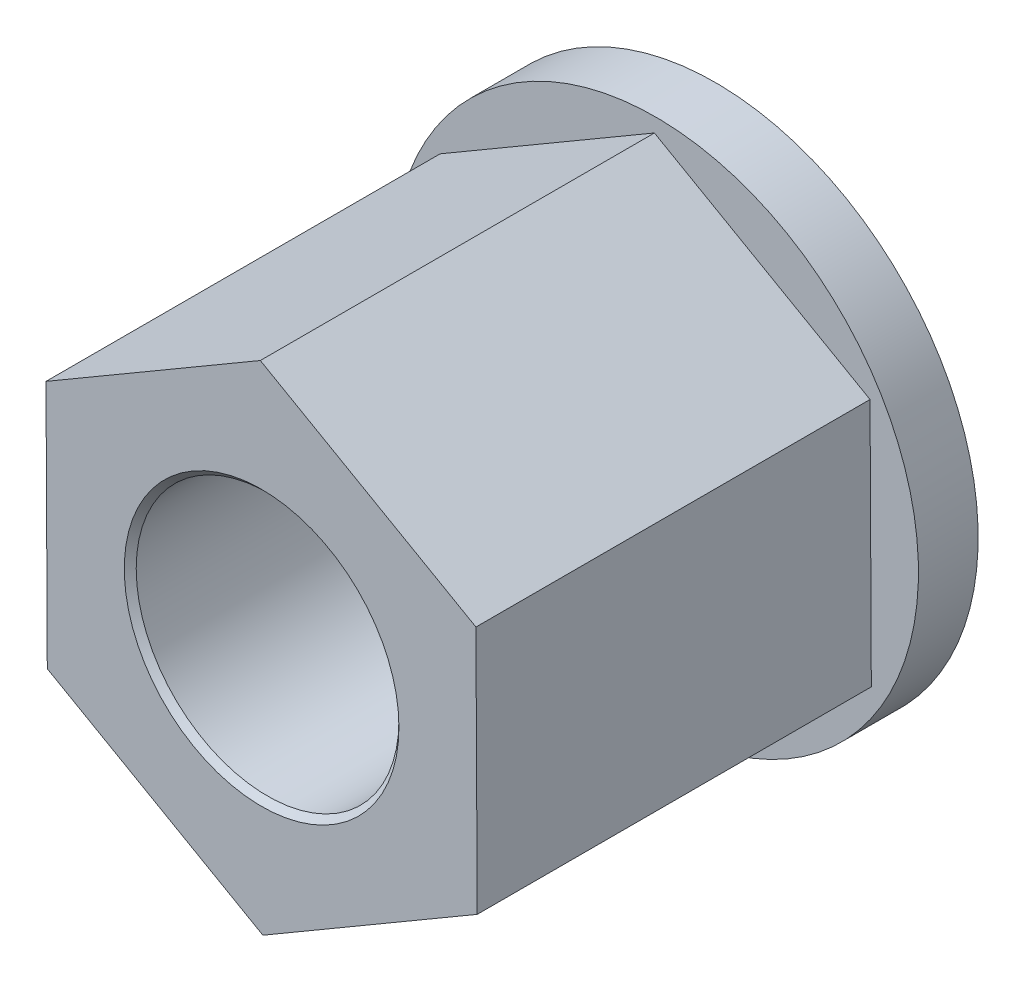
from build123d import *

# Parameters (mm, degrees)
SKETCH1_R                  = 22
BOSS_EXTRUDE_DEPTH         = 5
BOSS_EXTRUDE1_DEPTH        = 33
M24X2_0_TAPPED_HOLE1_D     = 22
M24X2_0_TAPPED_HOLE1_DEPTH = 58
M24X2_0_TAPPED_HOLE1_TIP   = 6.609466809
CHAMFER2_SIZE              = 0.5


with BuildPart() as part:
    # Sketch1 → Boss-Extrude (new body)
    with BuildSketch(Plane.XY):
        Circle(SKETCH1_R)
    extrude(amount=BOSS_EXTRUDE_DEPTH)

    # Sketch2 → Boss-Extrude1 (add)
    with BuildSketch(Plane.XY.offset(5)):
        Polygon((-17.945989557, -10.485297269), (0.107539023, -20.784331487), (18.05352858, -10.299034218), (17.945989557, 10.485297269), (-0.107539023, 20.784331487), (-18.05352858, 10.299034218), align=None)
    extrude(amount=BOSS_EXTRUDE1_DEPTH)

    # Sketch4 → Cut-Revolve1 (revolve, cut)
    with BuildSketch(Plane(origin=(0, 0, 0), x_dir=(0, 0, -1), z_dir=(1, 0, 0)), mode=Mode.PRIVATE) as cut_revolve1_sk:
        Polygon((-8.577004511, -2.997330388), (-6.875334866, -5.94470867), (-8.577004511, -5.94470867), align=None)
    revolve(cut_revolve1_sk.sketch.rotate(Axis((0, 0, 0), (0, 0, 1)), 270), axis=Axis((0, 0, 0), (0, 0, 1)), mode=Mode.SUBTRACT)

    # M24x2.0 Tapped Hole1
    with Locations(Plane.XY.offset(38)):
        with Locations((0, 0)):
            Hole(M24X2_0_TAPPED_HOLE1_D / 2, depth=M24X2_0_TAPPED_HOLE1_DEPTH)
            with Locations((0, 0, -(M24X2_0_TAPPED_HOLE1_DEPTH + M24X2_0_TAPPED_HOLE1_TIP / 2))):  # 118° drill point
                Cone(0, M24X2_0_TAPPED_HOLE1_D / 2, M24X2_0_TAPPED_HOLE1_TIP, mode=Mode.SUBTRACT)

    # Chamfer2
    chamfer2_edges = [part.edges().sort_by_distance(p)[0] for p in [
        (11, 0, 38),
    ]]
    chamfer(chamfer2_edges, length=CHAMFER2_SIZE)


solid = part.part
